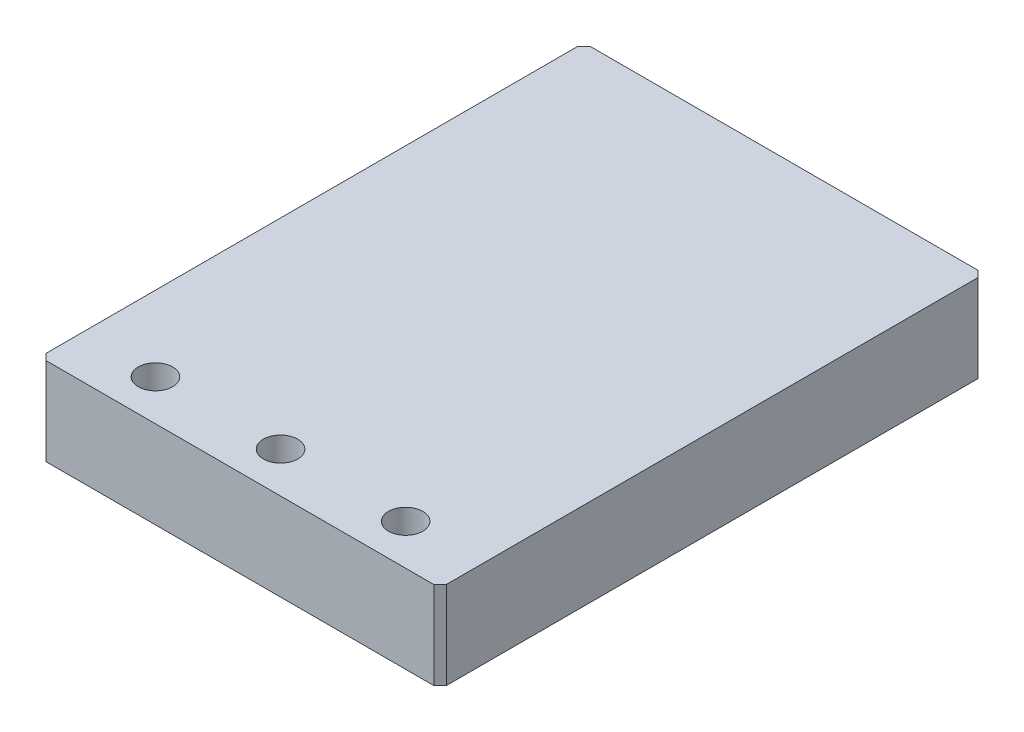
SolidWorks part; units mm, degrees
material "6061-T6 (SS)"
ref_plane "前视基准面" through (0, 0, 0) normal (0, 0, 1) x (1, 0, 0)
ref_plane "上视基准面" through (0, 0, 0) normal (0, 1, 0) x (1, 0, 0)
ref_plane "右视基准面" through (0, 0, 0) normal (1, 0, 0) x (0, 0, -1)
sketch "草图1" plane through (0, 0, 0) normal (0, 0, 1) x (1, 0, 0)
  line L1 (-22, -60.68) -> (42, -60.68)
  line L2 (-22, -60.68) -> (-22, -74.68)
  line L3 (-22, -74.68) -> (42, -74.68)
  line L4 (42, -60.68) -> (42, -74.68)
  dimension "D1" = 14
  dimension "D2" = 64
extrude "凸台-拉伸1" add sketch "草图1" along normal blind 87
hole_wizard "打孔尺寸根据六角头螺栓 C 级的类型0" positions "草图4" profile "草图2" counterbore size "M5" standard "Gb" end condition through all
sketch "草图4" plane through (0, -74.68, 0) normal (0, -1, 0) x (-1, 0, 0)
  line L0 (22, -87) -> (22, 0) construction
  line L2 (22, -87) -> (-42, -87) construction
  point P0 (10, -80.5)
  point P2 (-10, -80.5)
  point P4 (-30, -80.5)
  dimension "D1" = 12
  dimension "D2" = 20
  dimension "D3" = 20
  dimension "D4" = 6.5
sketch "草图2" plane through (-10, -74.68, 80.5) normal (1, 0, 0) x (0, 0, -1)
  line L0 (0, 0) -> (0, 14)
  line L1 (0, 14) -> (2.75, 14)
  line L3 (2.75, 14) -> (2.75, 5.5)
  line L4 (2.75, 5.5) -> (5, 5.5)
  line L5 (5, 5.5) -> (5, 0)
  line L7 (5, 0) -> (0, 0)
  line L11 (0, -6.35) -> (0, 107.95) construction
  dimension "通孔孔直径" = 5.5
  dimension "通孔孔深度" = 14
  dimension "柱形沉头孔直径" = 10
  dimension "柱形沉头孔深度" = 5.5
hole_wizard "M6 螺纹孔1" positions "草图6" profile "草图5" tap size "M6" standard "Iso"
sketch "草图6" plane through (0, 0, 0) normal (0, 0, -1) x (-1, 0, 0)
  line L0 (-42, -74.68) -> (-42, -60.68) construction
  line L1 (22, -74.68) -> (-42, -74.68) construction
  point P0 (-30, -67.68)
  point P2 (-10, -67.68)
  point P4 (10, -67.68)
  dimension "D1" = 12
  dimension "D2" = 20
  dimension "D3" = 20
  dimension "D4" = 7
sketch "草图5" plane through (30, -67.68, 0) normal (1, 0, 0) x (0, 1, 0)
  line L0 (0, 0) -> (0, 15.0022)
  line L1 (0, 15.0022) -> (2.5, 13.5)
  line L2 (2.5, 13.5) -> (2.5, 0)
  line L5 (2.5, 0) -> (0, 0)
  line L10 (0, 15.0022) -> (-2.5, 13.5) construction
  line L11 (0, -6.35) -> (0, 107.95) construction
  dimension "螺纹孔钻头直径" = 5
  dimension "螺纹孔钻头深度" = 13.5
  dimension "导头角度" = 118
cosmetic thread "孔螺蚊线1" parameters "D1"=12, "D2"=6
cosmetic thread "孔螺蚊线2" parameters "D1"=12, "D2"=6
cosmetic thread "孔螺蚊线3" parameters "D1"=12, "D2"=6
chamfer "倒角1" distance 1 angle 45 4 edges at (-22, -67.68, 87) (42, -67.68, 87) (-22, -67.68, 0) (42, -67.68, 0)
